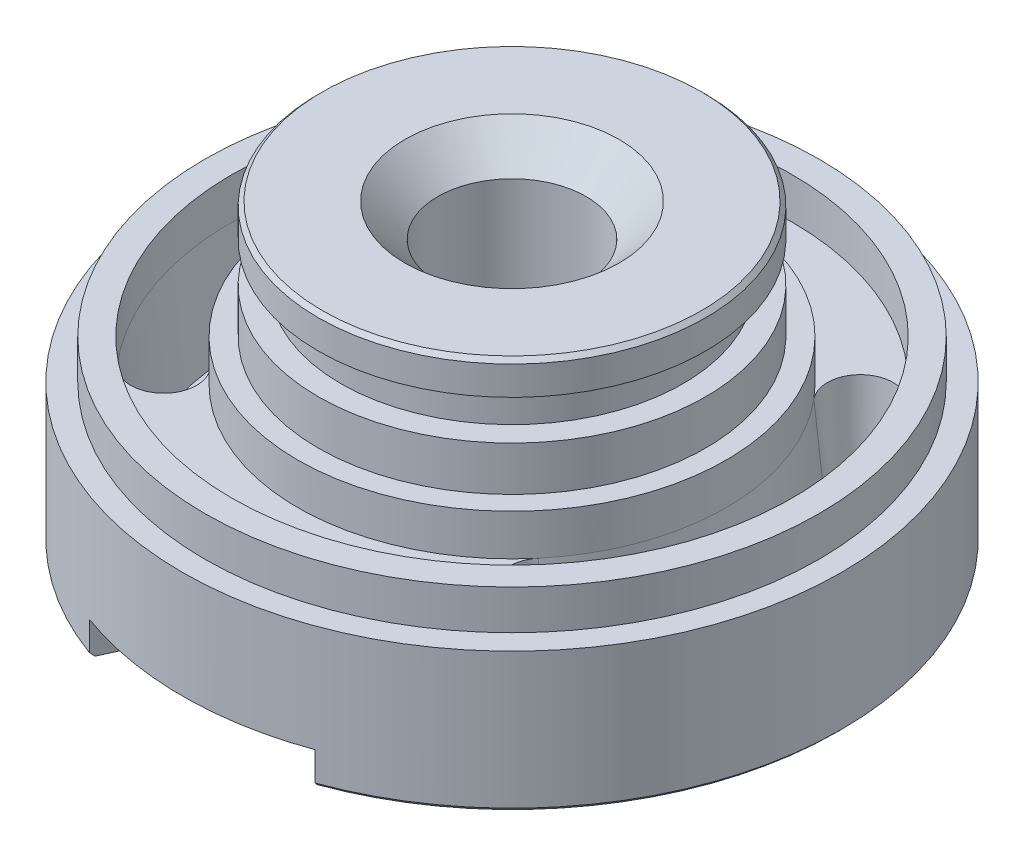
SolidWorks part; units mm, degrees
ref_plane "Front Plane" through (0, 0, 0) normal (0, 0, 1) x (1, 0, 0)
ref_plane "Top Plane" through (0, 0, 0) normal (0, 1, 0) x (1, 0, 0)
ref_plane "Right Plane" through (0, 0, 0) normal (1, 0, 0) x (0, 0, -1)
other "Configuration Table"
sketch "Sketch1" plane through (0, 0, 0) normal (0, 1, 0) x (1, 0, 0)
  circle A0 centre (0, 0) radius 40
  dimension "D1" = 80
extrude "Boss-Extrude1" add sketch "Sketch1" along normal blind 17
sketch "Sketch2" plane through (0, 17, 0) normal (0, 1, 0) x (1, 0, 0)
  circle A0 centre (0, 0) radius 37.26
  dimension "D1" = 74.52
extrude "Boss-Extrude2" add sketch "Sketch2" along normal blind 4.8
sketch "Sketch3" plane through (0, 21.8, 0) normal (0, 1, 0) x (1, 0, 0)
  circle A0 centre (0, 0) radius 23.5
  dimension "D1" = 47
extrude "Boss-Extrude3" add sketch "Sketch3" along normal blind 5.4
sketch "Sketch4" plane through (0, 27.2, 0) normal (0, 1, 0) x (1, 0, 0)
  circle A0 centre (0, 0) radius 20.76
  dimension "D1" = 41.52
extrude "Boss-Extrude4" add sketch "Sketch4" along normal blind 4.8
sketch "Sketch5" plane through (0, 32, 0) normal (0, 1, 0) x (1, 0, 0)
  circle A0 centre (0, 0) radius 23.5
  dimension "D1" = 47
extrude "Boss-Extrude5" add sketch "Sketch5" along normal blind 4
sketch "Sketch6" plane through (0, 36, 0) normal (0, 1, 0) x (1, 0, 0)
  circle A0 centre (0, 0) radius 9
  dimension "D1" = 18
extrude "Cut-Extrude1" cut sketch "Sketch6" against normal through all both and the other way through all
chamfer "Chamfer1" distance 4 angle 45 1 edges at (0, 36, 9)
sketch "Sketch7" plane through (0, 21.8, 0) normal (0, 1, 0) x (1, 0, 0)
  circle A0 centre (0, 0) radius 34
  circle A1 centre (0, 0) radius 26
  dimension "D1" = 68
  dimension "D2" = 52
extrude "Cut-Extrude2" cut sketch "Sketch7" against normal blind 5 and the other way through all
sketch "Sketch8" plane through (0, 0, 0) normal (0, -1, 0) x (-1, 0, 0)
  line L0 (0, 0) -> (0, -58.868) construction
  line L1 (47.3409, 0) -> (-47.3409, 0) construction
  line L2 (0, 0) -> (41.4328, -21.1111) construction
  line L3 (0, 0) -> (-41.4328, -21.1111) construction
  arc A0 (25.1624, -9.7906) -> (25.1624, 9.7906) centre (0, 0) ccw
  arc A2 (29.8073, -8.5161) -> (29.8073, 8.5161) centre (0, 0) ccw
  arc A3 (25.1624, -9.7906) -> (29.8073, -8.5161) centre (27.9582, -10.8784) ccw
  arc A4 (25.1624, 9.7906) -> (29.8073, 8.5161) centre (27.9582, 10.8784) cw
  arc A5 (-25.1624, 9.7906) -> (-29.8073, 8.5161) centre (-27.9582, 10.8784) ccw
  arc A6 (-25.1624, -9.7906) -> (-29.8073, -8.5161) centre (-27.9582, -10.8784) cw
  arc A7 (-29.8073, -8.5161) -> (-29.8073, 8.5161) centre (0, 0) cw
  arc A8 (-25.1624, -9.7906) -> (-25.1624, 9.7906) centre (0, 0) cw
  dimension "D1" = 54
  dimension "D2" = 62
  dimension "D4" = 6
  dimension "D3" = 27
extrude "Cut-Extrude3" cut sketch "Sketch8" against normal blind 4
sketch "Sketch9" plane through (0, 16.8, 0) normal (0, 1, 0) x (1, 0, 0)
  line L0 (-30, 0) -> (0, 0) construction
  arc A0 (-22.9813, -19.2836) -> (-22.9813, 19.2836) centre (0, 0) cw construction
  arc A1 (-26.0455, 21.8548) -> (-26.0455, -21.8548) centre (0, 0) ccw
  arc A2 (-19.9172, 16.7125) -> (-19.9172, -16.7125) centre (0, 0) ccw
  arc A3 (-19.9172, 16.7125) -> (-26.0455, 21.8548) centre (-22.9813, 19.2836) ccw
  arc A4 (-26.0455, -21.8548) -> (-19.9172, -16.7125) centre (-22.9813, -19.2836) ccw
  circle A5 centre (0, 0) radius 26 construction
  circle A6 centre (0, 0) radius 34 construction
  point P4 (-30, 0)
  dimension "D2" = 80
extrude "Cut-Extrude4" cut sketch "Sketch9" against normal up to surface (12.8 mm away) draft 5 contours A3 A1 A4 A2
mirror "Mirror1" about plane through (0, 0, 0) normal (1, 0, 0) of "Cut-Extrude4"
sketch "Sketch12" plane through (0, 0, 0) normal (0, -1, 0) x (-1, 0, 0)
  line L0 (0, -51.916) -> (0, 0) construction
  line L1 (36, 0) -> (-36, 0) construction
  point P3 (-36, 0)
  point P4 (36, 0)
  dimension "D1" = 36
hole_wizard "M4 Tapped Hole1" positions "Sketch12" profile "Sketch13" tap size "M4" standard "GB"
sketch "Sketch13" plane through (-36, 0, 0) normal (1, 0, 0) x (0, 0, -1)
  line L0 (0, 0) -> (0, 11.9914)
  line L1 (0, 11.9914) -> (1.65, 11)
  line L2 (1.65, 11) -> (1.65, 0.375)
  line L3 (1.65, 0.375) -> (2.025, 0)
  line L5 (2.025, 0) -> (0, 0)
  line L6 (-1.65, 0.375) -> (-2.025, 0) construction
  line L10 (0, 11.9914) -> (-1.65, 11) construction
  line L11 (0, -6.35) -> (0, 107.95) construction
  dimension "螺纹孔钻头直径" = 3.3
  dimension "螺纹孔钻头深度" = 11
  dimension "近端锥形沉头孔直径" = 4.05
  dimension "近端锥形沉头孔角度" = 90
  dimension "导头角度" = 118
cosmetic thread "Hole thread line 1" parameters "D1"=9, "D2"=4
cosmetic thread "Hole thread line 2" parameters "D1"=9, "D2"=4
sketch "Sketch14" plane through (0, 0, 0) normal (0, -1, 0) x (-1, 0, 0)
  line L0 (0, -53.1415) -> (0, 0) construction
  line L1 (0, 0) -> (67.5406, 0) construction
  line L2 (13.7004, -37.5806) -> (9.9772, -29.4109)
  line L3 (-13.7004, -37.5806) -> (-9.9772, -29.4109)
  line L4 (-13.7004, 37.5806) -> (-9.9772, 29.4109)
  line L5 (13.7004, 37.5806) -> (9.9772, 29.4109)
  arc A0 (-6.5571, -27.7354) -> (6.5571, -27.7354) centre (0, 0) ccw
  circle A1 centre (0, 0) radius 40 construction
  arc A2 (25.1624, -9.7906) -> (29.8073, -8.5161) centre (27.9582, -10.8784) ccw construction
  arc A3 (-13.7004, -37.5806) -> (13.7004, -37.5806) centre (0, 0) ccw
  arc A4 (-9.9772, -29.4109) -> (-6.5571, -27.7354) centre (-7.2474, -30.6549) cw
  arc A5 (9.9772, -29.4109) -> (6.5571, -27.7354) centre (7.2474, -30.6549) ccw
  arc A6 (9.9772, 29.4109) -> (6.5571, 27.7354) centre (7.2474, 30.6549) cw
  arc A7 (-9.9772, 29.4109) -> (-6.5571, 27.7354) centre (-7.2474, 30.6549) ccw
  arc A8 (-13.7004, 37.5806) -> (13.7004, 37.5806) centre (0, 0) cw
  arc A9 (-6.5571, 27.7354) -> (6.5571, 27.7354) centre (0, 0) cw
  point P15 (-8.9109, -27.0711)
  point P18 (8.9109, -27.0711)
  point P27 (8.9109, 27.0711)
  point P28 (-8.9109, 27.0711)
  dimension "D1" = 57
  dimension "D2" = 25
  dimension "D4" = 3
  dimension "D3" = 24.5
extrude "Cut-Extrude5" cut sketch "Sketch14" against normal blind 4
sketch "Sketch15" plane through (0, 0, 0) normal (0, -1, 0) x (-1, 0, 0)
  circle A0 centre (0, 0) radius 18.5
  circle A1 centre (0, 0) radius 14.5
  dimension "D1" = 37
  dimension "D2" = 29
extrude "Cut-Extrude6" cut sketch "Sketch15" against normal blind 3
chamfer "Chamfer2" distance 0.5 angle 45 3 edges at (-40, 0, 0) (40, 0, 0) (0, 36, 23.5)
